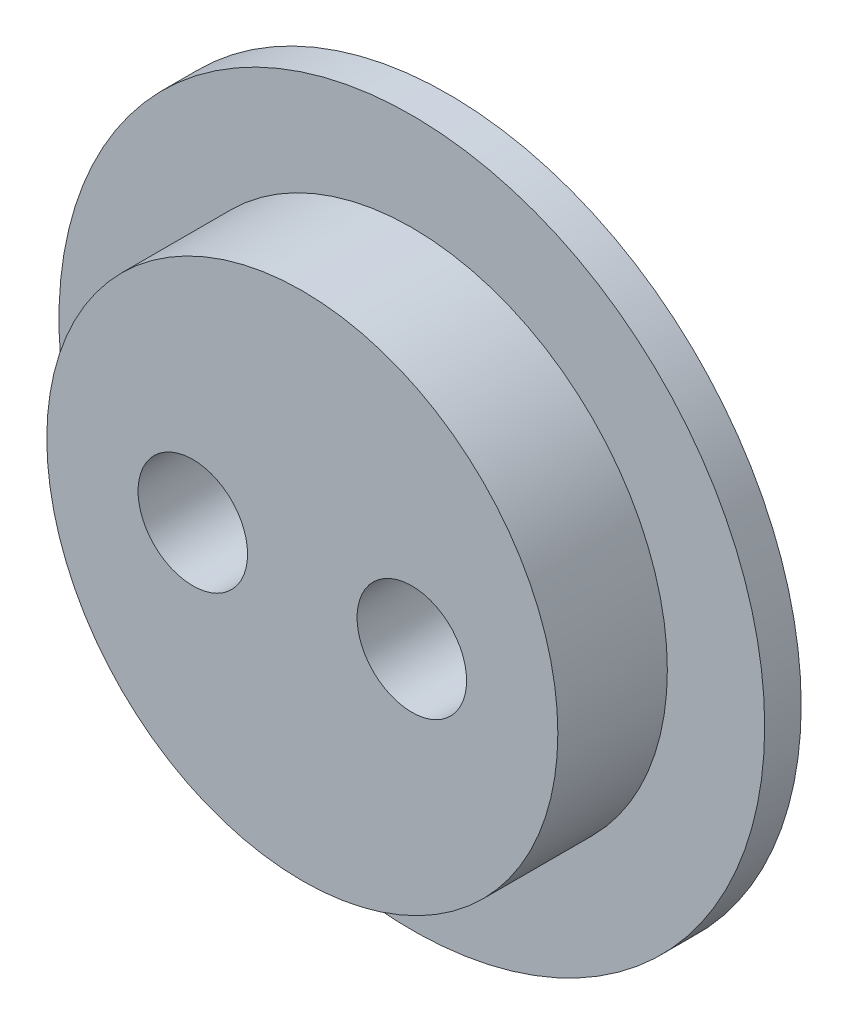
from build123d import *

# Parameters (mm, degrees)
SKETCH_1_R          = 29
EXTRUDE_1_DEPTH     = 3
SKETCH_2_R          = 21
EXTRUDE_2_DEPTH     = 9
SKETCH_3_R          = 4.5
CUT_EXTRUDE_1_DEPTH = 43.731721238


with BuildPart() as part:
    # 草图1 → 凸台-拉伸1 (new body)
    with BuildSketch(Plane.XY):
        Circle(SKETCH_1_R)
    extrude(amount=EXTRUDE_1_DEPTH)

    # 草图2 → 凸台-拉伸2 (add)
    with BuildSketch(Plane.XY.offset(3)):
        Circle(SKETCH_2_R)
    extrude(amount=EXTRUDE_2_DEPTH)

    # 草图3 → 切除-拉伸1 (cut, through all)
    with BuildSketch(Plane.XY.offset(12)):
        with Locations((-9, 0)):
            Circle(SKETCH_3_R)
        with Locations((9, 0)):
            Circle(SKETCH_3_R)
    extrude(amount=-CUT_EXTRUDE_1_DEPTH, mode=Mode.SUBTRACT)


solid = part.part
